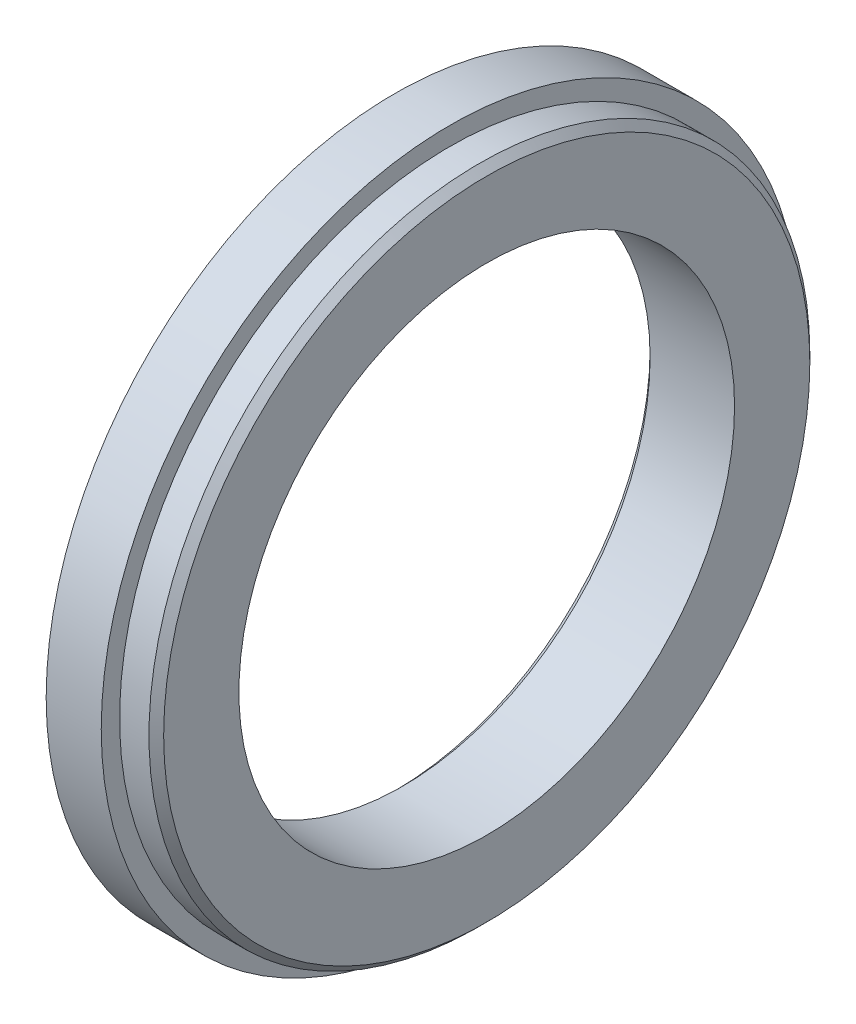
SolidWorks part; units mm, degrees
ref_plane "Front Plane" through (0, 0, 0) normal (0, 0, 1) x (1, 0, 0)
ref_plane "Top Plane" through (0, 0, 0) normal (0, 1, 0) x (1, 0, 0)
ref_plane "Right Plane" through (0, 0, 0) normal (1, 0, 0) x (0, 0, -1)
sketch "Sketch1" plane through (0, 0, 0) normal (1, 0, 0) x (0, 0, -1)
  circle A0 centre (0, 0) radius 95
  circle A1 centre (0, 0) radius 67.5
  dimension "D1" = 190
  dimension "D2" = 135
extrude "Boss-Extrude1" add sketch "Sketch1" along normal blind 25
sketch "Sketch2" plane through (25, 0, 0) normal (1, 0, 0) x (0, 0, -1)
  circle A0 centre (0, 0) radius 90
  circle A1 centre (0, 0) radius 95
  dimension "D1" = 180
extrude "Cut-Extrude1" cut sketch "Sketch2" against normal blind 10
sketch "Sketch3" plane through (0, 0, 0) normal (-1, 0, 0) x (0, 0, 1)
  circle A0 centre (40.25, -69.715) radius 5.75
  circle A1 centre (80.5, 0) radius 5.75
  circle A2 centre (-40.25, -69.715) radius 5.75
  circle A3 centre (-80.5, 0) radius 5.75
  circle A4 centre (-40.25, 69.715) radius 5.75
  circle A5 centre (40.25, 69.715) radius 5.75
  point P15 (0, 0)
  dimension "D1" = 6
  dimension "D2" = 11.5
extrude "Cut-Extrude2" cut sketch "Sketch3" against normal blind 17.5
chamfer "Chamfer1" distance 2 angle 45 2 edges at (0, 0, -67.5) (25, 0, -90)
